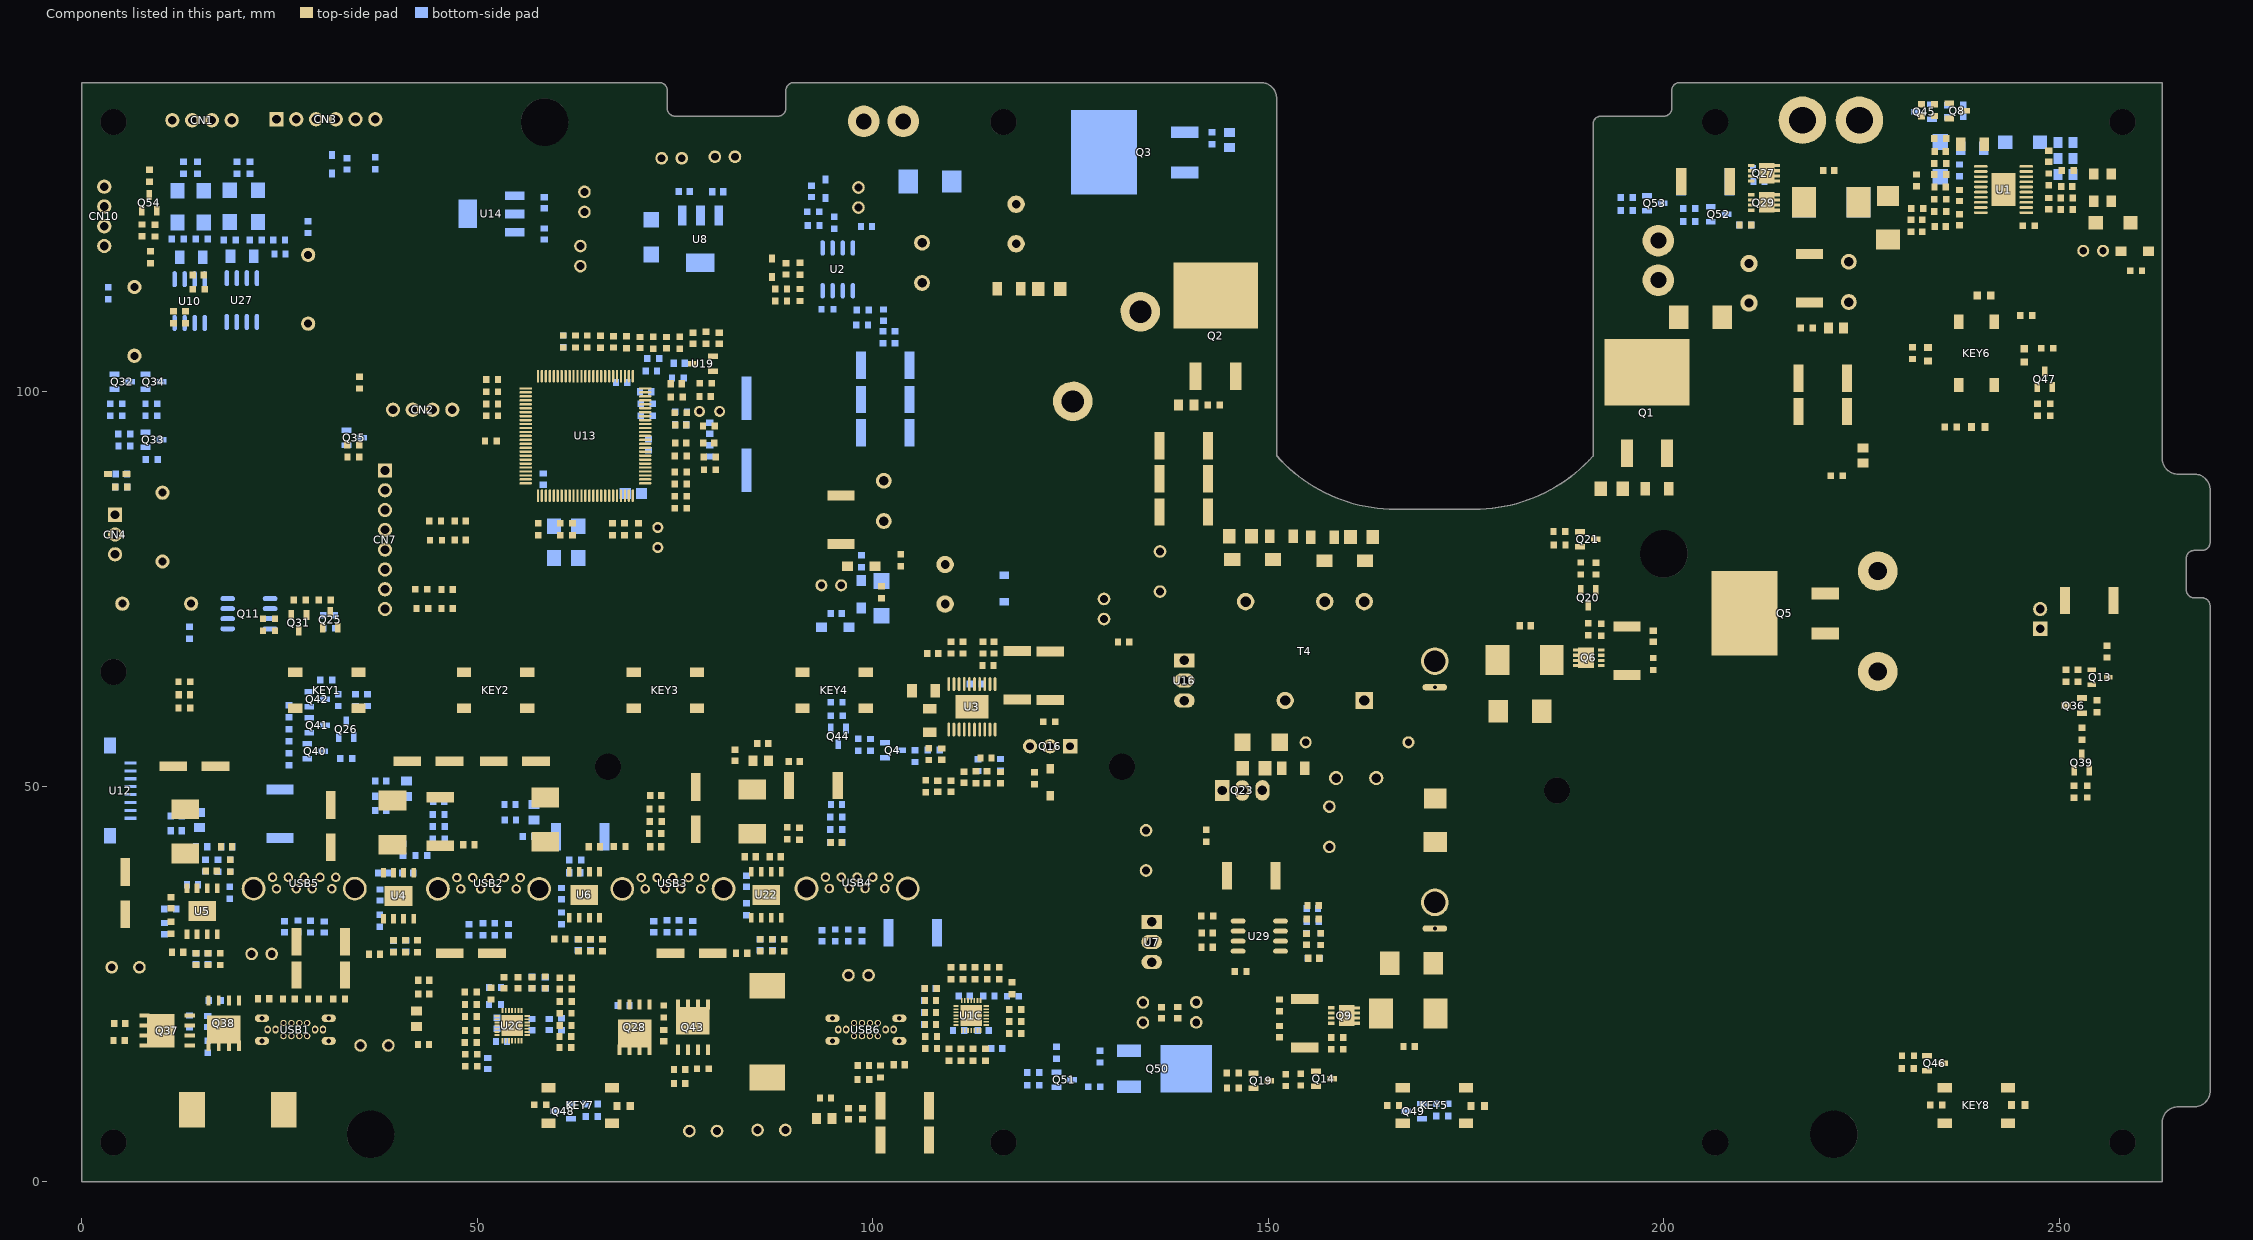
[diagram p0: the components of this part, seen from the top]
# Altium PCB MISC84402.PcbDoc (part 11 of 12)
Units mm, origin at the board's own origin, x right, y up, seen from the top; angles counter-clockwise.
Board outline 269.06 x 139 mm, 4 copper layers (TOP, GND02, PWR03, BOTTOM), stack 0.732 mm thick; 694 components, 428 nets, 1859 pads, 1384 vias.

## Polygon pours and split planes (outlines as drawn) (continued)
NETQ27_1 on BOTTOM "TOP-No Net 1" (solid, pour order 1486): 23 vertices, not listed, extent 206.965,123.317 211.963,129.286
NETC41_1 on BOTTOM "TOP-No Net 1" (solid, remove dead copper, pour order 1487): 219.837,137.287 220.472,136.652 220.472,122.428 219.837,121.793 215.138,121.793 214.21,122.721 214.21,136.359 215.138,137.287
B+ on BOTTOM "TOP-No Net 1" (solid, remove dead copper, pour order 1488): 30 vertices, not listed, extent 108.102,122.174 132.588,135.763
GND on BOTTOM "Bottom Layer-No Net 2" (solid, remove dead copper, pour order 1460): 93.345,127.508 98.679,127.508 99.06,127.127 99.06,125.222 98.552,124.714 96.139,124.714 95.377,125.476 92.329,125.476 92.202,125.603 92.202,127.254 92.456,127.508 93.345,127.508
BATA+ on BOTTOM "Bottom Layer-No Net 2" (solid, remove dead copper, pour order 1461): 102.743,125.095 105.791,125.095 106.426,125.73 106.426,129.413 106.68,129.667 109.728,129.667 110.49,130.429 110.49,138.43 110.236,138.684 102.489,138.684 101.854,138.049 101.854,125.349 102.108,125.095 102.235,124.968 102.489,124.968
GND on BOTTOM "Bottom Layer-No Net 2" (solid, remove dead copper, pour order 1462): 100.711,138.303 93.472,138.303 92.71,137.541 92.71,129.413 93.345,128.778 100.584,128.778 100.965,129.159 100.965,138.049 100.711,138.303
NETC33_1 on BOTTOM "BottomLayer-No Net" (solid, remove dead copper, pour order 1001): 55 vertices, not listed, extent 119.939,85.369 147.422,131.089
no net on DXF0111-TOP (solid): 259.402,3.812 259.361,3.765 259.241,3.912 259.402,3.812
no net on DXF0111-TOP (solid): 197.477,81.358 197.439,81.308 197.607,81.22 197.477,81.358
no net on DXF0111-TOP (solid): -32.786,0.187 -32.723,0.187 -32.754,0 -32.786,0.187
no net on DXF0111-TOP (solid): -32.786,138.812 -32.723,138.812 -32.754,139 -32.786,138.812
no net on DXF0111-TOP (solid): 262.813,165.978 262.813,165.916 263,165.947 262.813,165.978
no net on DXF0111-TOP (solid): 0.187,165.978 0.187,165.916 0,165.947 0.187,165.978

## Keep-outs
Keep-Out Layer:
  circle w0.025: c4,134 r4.75
  circle w0.025: c58.5,134 r5.5
  circle w0.025: c116.5,134 r5.258
  circle w0.025: c4,64.5 r4.75
  circle w0.025: c4.037,5.273 r4.75
  circle w0.025: c36.5,6.03 r6.008
  circle w0.025: c116.5,5 r5.258
  circle w0.025: c206.5,5 r5.004
  circle w0.025: c221.5,6.03 r5.004
  circle w0.025: c258,134 r5.004
  circle w0.025: c206.5,134 r5.004
  circle w0.025: c200,79.41 r5.754
  circle w0.025: c186.5,49.5 r5.004
  circle w0.025: c131.5,52.5 r5.258
  circle w0.025: c66.537,52.773 r4.75
  circle w0.025: c258,5 r5.004
  lines w0.025: 17.13,75.3 29.13,75.3 ; 17.13,105.3 29.13,105.3 ; 263,0 263,7.5 cw(c265,7.5) 265,9.5 267.058,9.5 ccw(c267.058,11.5) 269.058,11.5 269.058,72.85 ccw(c268.058,72.85) 268.058,73.85 267.058,73.85 cw(c267.058,74.85) 266.058,74.85 266.058,78.85 cw(c267.058,78.85) 267.058,79.85 268.058,79.85 ccw(c268.058,80.85) 269.058,80.85 269.058,87.5 ; 29.13,75.3 ccw(c29.13,77.3) 31.13,77.3 31.13,103.3 ccw(c29.13,103.3) 29.13,105.3 ; 29.13,75.3 15.13,75.3 cw(c15.13,77.3) 13.13,77.3 13.13,103.3 cw(c15.13,103.3) 15.13,105.3 29.13,105.3
  lines w0.127: 191.049,91.785 cw(c176.029,105.167) 176.029,85.05 166.081,85.05 cw(c166.081,105.12) 151.05,91.821 151.05,137 ccw(c149.05,137) 149.05,139 90,139 ccw(c90,138) 89,138 89,135.75 cw(c88,135.75) 88,134.75 75,134.75 cw(c75,135.75) 74,135.75 74,138 ccw(c73,138) 73,139 0,139 0,0 263,0 ; 191.05,91.785 191.05,133.75 cw(c192.05,133.75) 192.05,134.75 200,134.75 ccw(c200,135.75) 201,135.75 201,138 cw(c202,138) 202,139 263,139 263,91.5 ccw(c265,91.5) 265,89.5 267.058,89.5 cw(c267.058,87.5) 269.058,87.5

## Other copper
TOP:
  rectangle net +24V: 239.649,121.607 240.665,122.428
  rectangle net +24V: 6.477,17.11 11.949,21.844
  rectangle net NETQ5_3: 216.408,95.123 218.694,103.759
  rectangle net NETC10_1: 205.994,67.183 215.138,82.423
  rectangle net NETC10_1: 199.39,89.281 201.664,94.361
  rectangle net NETC10_1: 210.615,89.281 213.995,94.488
  rectangle net B+: 209.931,108.585 211.201,113.337
  rectangle net B+: 210.312,110.49 212.979,112.014
  rectangle net B+: 115.189,122.338 124.206,126.619
  rectangle net NETC41_1: 211.963,122.356 215.954,129.794
  rectangle net GND: 120.137,116.913 124.333,120.904
  rectangle net B+: 123.952,124.587 136.271,135.763
  rectangle net GND: 241.427,122.15 244.475,127.889
  rectangle net NETC33_1: 137.668,131.445 141.605,133.604
  rectangle net GND: 221.742,94.869 224.663,103.759
  rectangle net +13.6V: 226.441,117.348 230.251,120.777
  rectangle net GND: 200.254,124.409 203.835,128.473
  rectangle net VOUT2: 32.258,24.063 33.782,32.534
  rectangle net NETC77_1: 14.478,51.724 18.898,53.213
  rectangle net NETC77_1: 11.1,45.847 15.13,48.627
  rectangle net NetC3_2: 10.922,39.735 14.957,42.926
  rectangle net NetC3_2: 14.097,36.576 14.986,38.1
  rectangle net GND: 110.168,58.547 114.789,61.595
  rectangle net NetR54_1: 106.299,56.388 109.728,58.039
  rectangle net NETC33_1: 121.198,74.295 122.809,75.6
  rectangle net NETC33_1: 124.587,74.219 126.416,76.073
  rectangle net NETC33_1: 121.92,73.66 125.603,77.47
  rectangle net NETC33_1: 120.523,74.83 127.027,79.883
  rectangle net GND: 135.382,81.661 137.414,95.377
  rectangle net AGND: 45.136,51.968 47.752,54.331
  rectangle net AGND: 50.851,51.943 53.264,54.534
  rectangle net VBUSC-1: 101.24,18.11 102.002,19.269
  rectangle net +24V: 83.871,32.477 84.608,33.884
  rectangle net NetC8_2: 56.908,41.508 60.577,44.516
  rectangle net NETC115_1: 24.13,10.77 27.584,11.684
  rectangle net NETC115_1: 23.647,6.605 27.407,7.874
  rectangle net NETC115_1: 23.632,6.755 27.39,11.125
  rectangle net NETD62_2: 149.784,77.394 151.435,80.035
  rectangle net NETD62_2: 149.123,78.08 152.171,79.4
  rectangle net NETD62_2: 146.431,73.101 147.803,74.854
  rectangle net NETD62_2: 145.644,72.619 148.742,74.117
  rectangle net GND: 129.269,73.101 130.818,74.193
  rectangle net GND: 132.1,68.859 133.231,69.508
  rectangle net GND: 131.961,68.885 132.393,70.23
  rectangle net GND: 132.037,68.529 132.748,70.434
  rectangle net +12V: 138.514,59.309 140.37,60.655
  rectangle net +12V: 137.625,60.147 141.181,61.417
  rectangle net +12V: 128.634,69.596 129.868,71.069
  rectangle net +12V: 128.014,70.485 130.793,71.922
  rectangle net +VCC_BAT: 144.636,77.495 146.21,79.908
  rectangle net +VCC_BAT: 143.848,78.029 146.871,79.451
  rectangle net +VCC_BAT: 138.489,65.761 140.292,67.259
  rectangle net +VCC_BAT: 137.371,65.303 141.232,66.523
  rectangle net NETC49_2: 43.917,41.063 46.771,43.637
  rectangle net NETC49_2: 46.542,42.079 47.38,43.146
  rectangle net NETC95_1: 56.693,52.222 58.699,54.127
  rectangle net NETC95_1: 58.547,52.68 59.792,53.721
  rectangle net AGND: 76.657,43.459 78.588,45.669
  rectangle net AGND: 77.064,42.342 78.13,46.761
  rectangle net NETC199_2: 94.336,48.819 95.377,51.435
  rectangle net NETQ27_1: 209.169,123.317 211.455,125.222
  rectangle net NETQ27_1: 209.148,125.15 210.13,125.349
  rectangle net NETC41_1: 215.646,121.793 219.837,126.492
  rectangle net NETC41_2: 222.706,121.92 230.124,126.619
  rectangle net NETC41_2: 221.615,130.175 228.81,137.414
  rectangle net NETC41_2: 223.139,128.905 226.695,134.493
  rectangle net NETC41_1: 214.376,129.413 220.472,137.414
  rectangle net NETQ27_1: 209.296,127 211.455,129.286
  rectangle net B+: 124.333,124.587 135.001,135.763
  rectangle net GND: 120.396,118.237 123.19,120.904
  rectangle net +24V: 67.336,15.557 72.145,20.574
  rectangle net VBUSC-1: 96.176,18.047 96.938,19.206
  rectangle net VBUSC-1: 105.918,3.429 108.458,12.319
  rectangle net VOUT1: 100.084,3.342 102.362,11.684
  rectangle net BATA+: 102.235,131.318 105.283,136.779
  rectangle net BATA+: 104.267,132.715 106.934,135.255
  rectangle net GND: 97.409,131.064 100.33,136.652
  rectangle net GND: 95.885,132.969 98.679,135.382
  pour cut-out: 89.733,6.569 89.706,6.778 89.625,6.972 89.497,7.14 89.33,7.268 89.135,7.348 88.926,7.376 88.717,7.348 88.522,7.268 88.355,7.14 88.227,6.972 88.146,6.778 88.119,6.569 88.146,6.36 88.227,6.165 88.355,5.998 88.522,5.87 88.717,5.789 88.926,5.761 89.135,5.789 89.33,5.87 89.497,5.998 89.625,6.165 89.706,6.36
  pour cut-out: 14.868,73.117 14.832,73.392 14.726,73.648 14.557,73.868 14.337,74.036 14.081,74.142 13.806,74.179 13.531,74.142 13.275,74.036 13.055,73.868 12.886,73.648 12.78,73.392 12.744,73.117 12.78,72.842 12.886,72.586 13.055,72.366 13.275,72.197 13.531,72.091 13.806,72.055 14.081,72.091 14.337,72.197 14.557,72.366 14.726,72.586 14.832,72.842
  pour cut-out: 11.248,78.451 11.212,78.726 11.106,78.982 10.937,79.202 10.717,79.37 10.461,79.476 10.186,79.513 9.911,79.476 9.655,79.37 9.435,79.202 9.266,78.982 9.16,78.726 9.124,78.451 9.16,78.176 9.266,77.92 9.435,77.7 9.655,77.531 9.911,77.425 10.186,77.389 10.461,77.425 10.717,77.531 10.937,77.7 11.106,77.92 11.212,78.176
  pour cut-out: 11.094,87.151 11.063,87.386 10.972,87.605 10.828,87.793 10.64,87.937 10.421,88.028 10.186,88.059 9.951,88.028 9.732,87.937 9.544,87.793 9.399,87.605 9.309,87.386 9.278,87.151 9.309,86.916 9.399,86.697 9.544,86.509 9.732,86.364 9.951,86.273 10.186,86.243 10.421,86.273 10.64,86.364 10.828,86.509 10.972,86.697 11.063,86.916
  pour cut-out: 169.899,62.949 172.2,62.949 172.234,62.947 172.269,62.942 172.303,62.935 172.336,62.924 172.369,62.911 172.4,62.895 172.429,62.876 172.457,62.855 172.483,62.831 172.506,62.805 172.527,62.778 172.546,62.748 172.562,62.717 172.576,62.685 172.586,62.652 172.594,62.618 172.598,62.583 172.6,62.548 172.598,62.513 172.593,62.479 172.586,62.444 172.575,62.411 172.562,62.379 172.546,62.348 172.527,62.318 172.506,62.291 172.482,62.265 172.456,62.241 172.429,62.22 172.399,62.201 172.368,62.185 172.336,62.172 172.303,62.162 172.269,62.154 172.234,62.149 172.2,62.148 169.899,62.148 169.864,62.15 169.83,62.154 169.796,62.162 169.762,62.172 169.73,62.186 169.699,62.202 169.67,62.22 169.642,62.242 169.616,62.265 169.593,62.291 169.572,62.319 169.553,62.348 169.537,62.379 169.523,62.412 169.513,62.445 169.505,62.479 169.501,62.514 169.499,62.549 169.501,62.583 169.505,62.618 169.513,62.652 169.524,62.685 169.537,62.718 169.553,62.749 169.572,62.778 169.593,62.806 169.617,62.831 169.642,62.855 169.67,62.876 169.7,62.895 169.731,62.911 169.763,62.925 169.796,62.935 169.83,62.943 169.865,62.947
  pour cut-out: 169.899,31.648 169.864,31.65 169.83,31.654 169.795,31.662 169.762,31.672 169.73,31.686 169.699,31.702 169.669,31.721 169.642,31.742 169.616,31.765 169.592,31.791 169.571,31.819 169.552,31.848 169.536,31.879 169.523,31.912 169.512,31.945 169.505,31.979 169.5,32.014 169.499,32.048 169.5,32.083 169.505,32.118 169.512,32.152 169.523,32.185 169.536,32.218 169.552,32.249 169.571,32.278 169.592,32.306 169.616,32.332 169.642,32.355 169.669,32.376 169.699,32.395 169.73,32.411 169.762,32.425 169.795,32.435 169.83,32.443 169.864,32.447 169.899,32.449 172.199,32.449 172.234,32.447 172.269,32.443 172.303,32.435 172.336,32.425 172.368,32.411 172.399,32.395 172.429,32.376 172.457,32.355 172.482,32.332 172.506,32.306 172.527,32.278 172.546,32.249 172.562,32.218 172.575,32.185 172.586,32.152 172.594,32.118 172.598,32.083 172.6,32.048 172.598,32.014 172.594,31.979 172.586,31.945 172.575,31.912 172.562,31.879 172.546,31.848 172.527,31.819 172.506,31.791 172.482,31.765 172.457,31.742 172.429,31.721 172.399,31.702 172.368,31.686 172.336,31.672 172.303,31.662 172.269,31.654 172.234,31.65 172.199,31.648
  pour cut-out: 59.877,120.552 59.845,120.711 59.755,120.846 59.621,120.936 59.462,120.967 59.303,120.936 59.169,120.846 59.079,120.711 59.047,120.552 59.079,120.394 59.169,120.259 59.303,120.169 59.462,120.138 59.621,120.169 59.755,120.259 59.845,120.394
  pour cut-out: 161.124,61.871 163.125,61.871 163.125,59.871 161.124,59.871
  pour cut-out: 164.384,51.095 164.356,51.304 164.276,51.499 164.147,51.666 163.98,51.794 163.785,51.875 163.577,51.902 163.368,51.875 163.173,51.794 163.006,51.666 162.877,51.499 162.797,51.304 162.769,51.095 162.797,50.886 162.877,50.691 163.006,50.524 163.173,50.396 163.368,50.315 163.577,50.288 163.785,50.315 163.98,50.396 164.147,50.524 164.276,50.691 164.356,50.886
  pour cut-out: 77.597,6.442 77.57,6.651 77.489,6.845 77.361,7.013 77.193,7.141 76.999,7.221 76.79,7.249 76.581,7.221 76.386,7.141 76.219,7.013 76.091,6.845 76.01,6.651 75.983,6.442 76.01,6.233 76.091,6.038 76.219,5.871 76.386,5.743 76.581,5.662 76.79,5.634 76.999,5.662 77.193,5.743 77.361,5.871 77.489,6.038 77.57,6.233
  pour cut-out: 8.072,27.143 8.045,27.352 7.964,27.546 7.836,27.714 7.669,27.842 7.474,27.922 7.265,27.95 7.056,27.922 6.861,27.842 6.694,27.714 6.566,27.546 6.485,27.352 6.458,27.143 6.485,26.934 6.566,26.739 6.694,26.572 6.861,26.444 7.056,26.363 7.265,26.335 7.474,26.363 7.669,26.444 7.836,26.572 7.964,26.739 8.045,26.934
  pour cut-out: 81.097,6.442 81.07,6.651 80.989,6.845 80.861,7.013 80.694,7.141 80.499,7.221 80.29,7.249 80.081,7.221 79.886,7.141 79.719,7.013 79.591,6.845 79.51,6.651 79.483,6.442 79.51,6.233 79.591,6.038 79.719,5.871 79.886,5.743 80.081,5.662 80.29,5.634 80.499,5.662 80.694,5.743 80.861,5.871 80.989,6.038 81.07,6.233
  pour cut-out: 144.473,70.929 143.838,70.294 143.838,64.198 144.219,63.817 164.793,63.817 165.174,64.198 165.174,70.421 164.666,70.929
GND02:
  rectangle net B+: 114.935,122.809 120.827,126.619
  rectangle net GND: 97.565,131.216 100.054,137.058
  rectangle net GND: 95.584,132.69 101.219,135.56
  rectangle net GND: 98.171,115.57 100.965,119.761
  pour cut-out: 243.112,112.395 243.08,112.554 242.99,112.688 242.856,112.778 242.697,112.81 242.538,112.778 242.404,112.688 242.314,112.554 242.282,112.395 242.314,112.236 242.404,112.102 242.538,112.012 242.697,111.98 242.856,112.012 242.99,112.102 243.08,112.236
  pour cut-out: 253.145,124.398 253.113,124.557 253.023,124.691 252.889,124.781 252.73,124.813 252.571,124.781 252.437,124.691 252.347,124.557 252.315,124.398 252.347,124.239 252.437,124.105 252.571,124.015 252.73,123.983 252.889,124.015 253.023,124.105 253.113,124.239
  pour cut-out: 114.334,69.215 114.302,69.374 114.212,69.508 114.078,69.598 113.919,69.63 113.76,69.598 113.626,69.508 113.536,69.374 113.504,69.215 113.536,69.056 113.626,68.922 113.76,68.832 113.919,68.8 114.078,68.832 114.212,68.922 114.302,69.056
  pour cut-out: 125.432,121.793 125.73,122.091 125.73,123.444 126.619,124.333 133.985,124.333 135.001,125.349 135.001,140.589 133.731,141.859 108.61,141.859 106.02,139.268 106.02,124.612 108.839,121.793
  pour cut-out: 135.154,137.287 145.923,137.287 147.193,136.017 152.4,101.981 146.808,101.977 144.149,101.977 143.891,102.235 144.145,102.489 144.145,135.89 143.764,136.271 136.144,136.271 135.001,135.128 134.147,135.128 133.858,135.417 133.858,135.991
  pour cut-out: 126.873,102.235 125.603,103.505 125.603,123.444 126.238,124.079 133.731,124.079 135.001,125.349 135.001,135.89 134.62,136.271 134.138,136.271 133.858,135.991 133.858,125.476 133.35,124.968 125.302,124.968 124.333,123.999 124.333,102.743 126.111,100.965 146.939,100.965 147.193,101.219 147.066,101.346 147.066,102.108 146.939,102.235
  pour cut-out: 136.77,52.5 136.725,53.188 136.59,53.864 136.369,54.516 136.064,55.135 135.681,55.708 135.226,56.226 134.708,56.681 134.135,57.064 133.517,57.368 132.864,57.59 132.188,57.725 131.5,57.77 130.812,57.725 130.136,57.59 129.483,57.368 128.865,57.064 128.292,56.681 127.774,56.226 127.319,55.708 126.936,55.135 126.631,54.516 126.41,53.864 126.275,53.188 126.23,52.5 126.275,51.812 126.41,51.136 126.631,50.483 126.936,49.865 127.319,49.292 127.774,48.773 128.292,48.319 128.865,47.936 129.483,47.631 130.136,47.409 130.812,47.275 131.5,47.23 132.188,47.275 132.864,47.409 133.517,47.631 134.135,47.936 134.708,48.319 135.226,48.773 135.681,49.292 136.064,49.865 136.369,50.483 136.59,51.136 136.725,51.812
  pour cut-out: 191.515,49.5 191.472,50.154 191.344,50.798 191.133,51.419 190.843,52.007 190.479,52.553 190.046,53.046 189.553,53.478 189.008,53.843 188.419,54.133 187.798,54.344 187.155,54.472 186.5,54.515 185.845,54.472 185.202,54.344 184.581,54.133 183.992,53.843 183.447,53.478 182.954,53.046 182.521,52.553 182.157,52.007 181.867,51.419 181.656,50.798 181.528,50.154 181.485,49.5 181.528,48.845 181.656,48.202 181.867,47.581 182.157,46.992 182.521,46.447 182.954,45.954 183.447,45.521 183.992,45.157 184.581,44.866 185.202,44.656 185.845,44.528 186.5,44.485 187.155,44.528 187.798,44.656 188.419,44.866 189.008,45.157 189.553,45.521 190.046,45.954 190.479,46.447 190.843,46.992 191.133,47.581 191.344,48.202 191.472,48.845
  pour cut-out: 205.767,79.41 205.717,80.163 205.57,80.902 205.328,81.617 204.994,82.293 204.575,82.921 204.078,83.488 203.511,83.985 202.883,84.404 202.207,84.738 201.492,84.98 200.753,85.127 200,85.177 199.247,85.127 198.507,84.98 197.793,84.738 197.116,84.404 196.489,83.985 195.922,83.488 195.425,82.921 195.006,82.293 194.672,81.617 194.429,80.902 194.282,80.163 194.233,79.41 194.282,78.657 194.429,77.917 194.672,77.203 195.006,76.526 195.425,75.899 195.922,75.332 196.489,74.835 197.116,74.415 197.793,74.082 198.507,73.839 199.247,73.692 200,73.643 200.753,73.692 201.492,73.839 202.207,74.082 202.883,74.415 203.511,74.835 204.078,75.332 204.575,75.899 204.994,76.526 205.328,77.203 205.57,77.917 205.717,78.657
  pour cut-out: 226.515,6.03 226.472,6.685 226.344,7.328 226.133,7.949 225.843,8.538 225.479,9.083 225.046,9.576 224.553,10.009 224.008,10.373 223.419,10.663 222.798,10.874 222.155,11.002 221.5,11.045 220.845,11.002 220.202,10.874 219.581,10.663 218.992,10.373 218.447,10.009 217.954,9.576 217.521,9.083 217.157,8.538 216.866,7.949 216.656,7.328 216.528,6.685 216.485,6.03 216.528,5.375 216.656,4.732 216.866,4.111 217.157,3.522 217.521,2.977 217.954,2.484 218.447,2.051 218.992,1.687 219.581,1.396 220.202,1.186 220.845,1.058 221.5,1.015 222.155,1.058 222.798,1.186 223.419,1.396 224.008,1.687 224.553,2.051 225.046,2.484 225.479,2.977 225.843,3.522 226.133,4.111 226.344,4.732 226.472,5.375
  pour cut-out: 2.705,0.51 0.51,0.51 0.51,1.848 0.511,1.857 0.513,1.866 0.516,1.874 0.519,1.882 0.523,1.89 0.528,1.897 0.534,1.904 0.54,1.911 0.546,1.917 0.553,1.922 0.561,1.927 0.569,1.931 0.577,1.934 0.586,1.936 0.594,1.938 0.603,1.939 0.612,1.94 0.621,1.939 0.63,1.938 0.638,1.936 0.647,1.933 0.655,1.929 0.663,1.925 0.67,1.92 0.677,1.915 0.682,1.91 0.988,1.63 1.317,1.378 1.667,1.156 2.035,0.965 2.418,0.807 2.723,0.708 2.731,0.705 2.739,0.702 2.747,0.698 2.755,0.693 2.762,0.687 2.768,0.681 2.774,0.674 2.779,0.667 2.784,0.66 2.788,0.652 2.791,0.643 2.793,0.635 2.795,0.626 2.796,0.617 2.796,0.609 2.796,0.6 2.794,0.591 2.792,0.582 2.789,0.574 2.786,0.566 2.782,0.558 2.777,0.551 2.771,0.544 2.765,0.537 2.758,0.532 2.751,0.526 2.744,0.522 2.736,0.518 2.728,0.514 2.719,0.512 2.71,0.51
  pour cut-out: 262.49,136.598 262.489,136.589 262.487,136.58 262.484,136.572 262.481,136.564 262.477,136.556 262.472,136.549 262.466,136.542 262.46,136.535 262.454,136.529 262.447,136.524 262.439,136.519 262.431,136.515 262.423,136.512 262.414,136.51 262.406,136.508 262.397,136.507 262.388,136.506 262.379,136.507 262.37,136.508 262.362,136.51 262.353,136.513 262.345,136.517 262.337,136.521 262.33,136.526 262.323,136.531 262.317,136.537 262.311,136.544 262.305,136.551 262.302,136.556 262.063,136.922 261.793,137.265 261.494,137.583 261.168,137.874 260.819,138.135 260.556,138.302 260.549,138.307 260.542,138.312 260.535,138.318 260.529,138.325 260.524,138.332 260.519,138.34 260.515,138.348 260.512,138.356 260.51,138.364 260.508,138.373 260.507,138.382 260.506,138.391 260.507,138.399 260.508,138.408 260.51,138.417 260.513,138.425 260.516,138.433 260.521,138.441 260.526,138.449 260.531,138.456 260.537,138.462 260.544,138.468 260.551,138.473 260.558,138.478 260.566,138.482 260.574,138.485 260.583,138.488 260.592,138.49 260.598,138.49 262.49,138.49
  pour cut-out: 127.929,39.895 123.456,39.895 123.329,39.768 123.329,33.495 127.929,33.495
  pour cut-out: 134.533,39.895 130.06,39.895 129.933,39.768 129.933,33.495 134.533,33.495
  pour cut-out: 144.473,70.929 143.838,70.294 143.838,64.198 144.219,63.817 164.793,63.817 165.174,64.198 165.174,70.421 164.666,70.929
  pour cut-out: 108.61,141.859 102.362,141.859 101.219,140.716 101.219,132.715 103.632,130.302 105.664,130.302 105.664,130.175 106.172,129.667 106.172,129.921 108.61,132.359